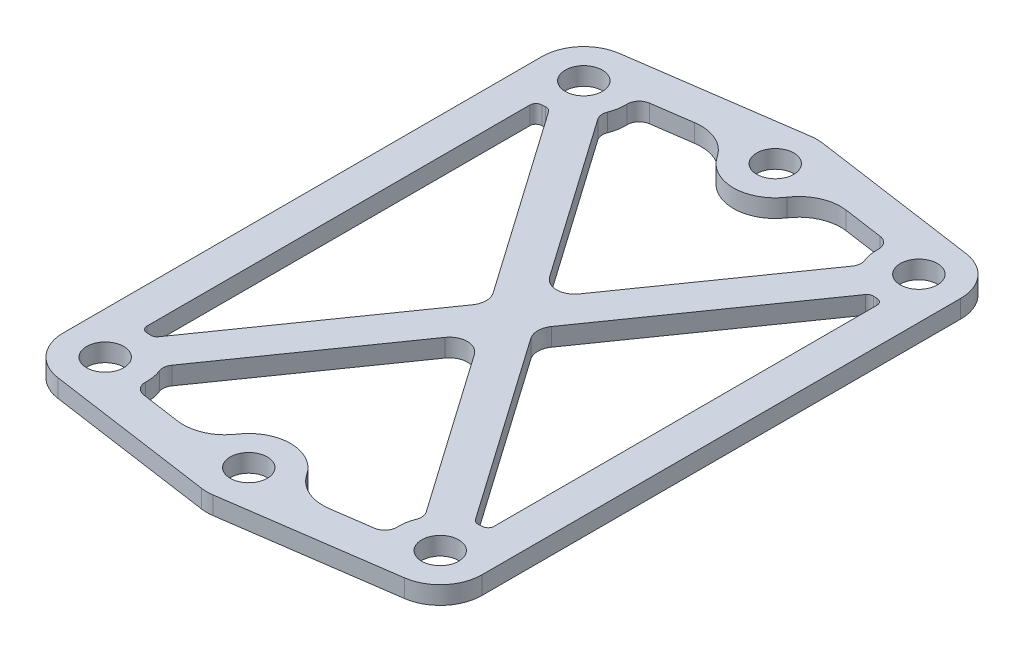
from build123d import *

# Parameters (mm, degrees)
SKETCH_1_R      = 1.55
EXTRUDE_1_DEPTH = 1.5
FILLET_1_R      = 0.5
FILLET_2_R      = 1
FILLET_3_R      = 1.5
FILLET_4_R      = 3.5


with BuildPart() as part:
    # 草图1 → 凸台-拉伸1 (new body)
    with BuildSketch(Plane(origin=(0, 0, 0), x_dir=(1, 0, 0), z_dir=(0, 1, 0))):
        with BuildLine():
            ThreePointArc((14.494974747, -23.464823228), (16.644088842, -22.293206095), (17.5, -20))
            Line((17.5, -20), (17.5, 20))
            ThreePointArc((17.5, 20), (16.644088842, 22.293206095), (14.494974747, 23.464823228))
            Line((14.494974747, 23.464823228), (0.494974747, 25.464823228))
            ThreePointArc((0.494974747, 25.464823228), (0, 25.5), (-0.494974747, 25.464823228))
            Line((-0.494974747, 25.464823228), (-14.494974747, 23.464823228))
            ThreePointArc((-14.494974747, 23.464823228), (-16.644088842, 22.293206095), (-17.5, 20))
            Line((-17.5, 20), (-17.5, -20))
            ThreePointArc((-17.5, -20), (-16.644088842, -22.293206095), (-14.494974747, -23.464823228))
            Line((-14.494974747, -23.464823228), (-0.494974747, -25.464823228))
            ThreePointArc((-0.494974747, -25.464823228), (0, -25.5), (0.494974747, -25.464823228))
            Line((0.494974747, -25.464823228), (14.494974747, -23.464823228))
        make_face()
        with BuildLine():
            Line((-10.957704959, -18.269554716), (0, -2.615690489))
            Line((0, -2.615690489), (10.957704959, -18.269554716))
            ThreePointArc((10.957704959, -18.269554716), (10.523504332, -19.595058191), (10.641425038, -20.984872695))
            Line((10.641425038, -20.984872695), (3.499996318, -22.005076798))
            ThreePointArc((3.499996318, -22.005076798), (0, -18.5), (-3.499996318, -22.005076798))
            Line((-3.499996318, -22.005076798), (-10.641425038, -20.984872695))
            ThreePointArc((-10.641425038, -20.984872695), (-10.523504332, -19.595058191), (-10.957704959, -18.269554716))
        make_face(mode=Mode.SUBTRACT)
        with BuildLine():
            ThreePointArc((14.5, -16.535898385), (13.957183203, -16.500261907), (13.41540072, -16.549167683))
            Line((13.41540072, -16.549167683), (1.830983342, 0))
            Line((1.830983342, 0), (13.41540072, 16.549167683))
            ThreePointArc((13.41540072, 16.549167683), (13.957183203, 16.500261907), (14.5, 16.535898385))
            Line((14.5, 16.535898385), (14.5, -16.535898385))
        make_face(mode=Mode.SUBTRACT)
        with BuildLine():
            Line((10.957704959, 18.269554716), (0, 2.615690489))
            Line((0, 2.615690489), (-10.957704959, 18.269554716))
            ThreePointArc((-10.957704959, 18.269554716), (-10.523504332, 19.595058191), (-10.641425038, 20.984872695))
            Line((-10.641425038, 20.984872695), (-3.499996318, 22.005076798))
            ThreePointArc((-3.499996318, 22.005076798), (0, 18.5), (3.499996318, 22.005076798))
            Line((3.499996318, 22.005076798), (10.641425038, 20.984872695))
            ThreePointArc((10.641425038, 20.984872695), (10.523504332, 19.595058191), (10.957704959, 18.269554716))
        make_face(mode=Mode.SUBTRACT)
        with Locations(Location((-14, -20, 0), (0, 0, 270))):
            Circle(SKETCH_1_R, mode=Mode.SUBTRACT)
        with BuildLine():
            Line((-1.830983342, 0), (-13.41540072, -16.549167683))
            ThreePointArc((-13.41540072, -16.549167683), (-13.957183203, -16.500261907), (-14.5, -16.535898385))
            Line((-14.5, -16.535898385), (-14.5, 16.535898385))
            ThreePointArc((-14.5, 16.535898385), (-13.957183203, 16.500261907), (-13.41540072, 16.549167683))
            Line((-13.41540072, 16.549167683), (-1.830983342, 0))
        make_face(mode=Mode.SUBTRACT)
        with Locations(Location((-14, 20, 0), (0, 0, 270))):
            Circle(SKETCH_1_R, mode=Mode.SUBTRACT)
        with Locations(Location((0, 22, 0), (0, 0, 270))):
            Circle(SKETCH_1_R, mode=Mode.SUBTRACT)
        with Locations(Location((0, -22, 0), (0, 0, 270))):
            Circle(SKETCH_1_R, mode=Mode.SUBTRACT)
        with Locations(Location((14, -20, 0), (0, 0, 270))):
            Circle(SKETCH_1_R, mode=Mode.SUBTRACT)
        with Locations(Location((14, 20, 0), (0, 0, 270))):
            Circle(SKETCH_1_R, mode=Mode.SUBTRACT)
    extrude(amount=EXTRUDE_1_DEPTH)

    # 圆角1
    fillet_1_edges = [part.edges().sort_by_distance(p)[0] for p in [
        (-14.5, 0.75, -16.535898385),
        (-14.5, 0.75, 16.535898385),
        (-13.41540072, 0.75, 16.549167683),
        (-13.41540072, 0.75, -16.549167683),
        (13.41540072, 0.75, 16.549167683),
        (14.5, 0.75, 16.535898385),
        (14.5, 0.75, -16.535898385),
        (13.41540072, 0.75, -16.549167683),
    ]]
    fillet(fillet_1_edges, radius=FILLET_1_R)

    # 圆角2
    fillet_2_edges = [part.edges().sort_by_distance(p)[0] for p in [
        (-10.957704959, 0.75, 18.269554716),
        (-10.641425038, 0.75, 20.984872695),
        (10.641425038, 0.75, 20.984872695),
        (10.957704959, 0.75, 18.269554716),
        (-10.641425038, 0.75, -20.984872695),
        (-10.957704959, 0.75, -18.269554716),
        (10.957704959, 0.75, -18.269554716),
        (10.641425038, 0.75, -20.984872695),
    ]]
    fillet(fillet_2_edges, radius=FILLET_2_R)

    # 圆角3
    fillet_3_edges = [part.edges().sort_by_distance(p)[0] for p in [
        (-1.830983342, 0.75, 0),
        (0, 0.75, 2.615690489),
        (1.830983342, 0.75, 0),
        (0, 0.75, -2.615690489),
    ]]
    fillet(fillet_3_edges, radius=FILLET_3_R)

    # 圆角4
    fillet_4_edges = [part.edges().sort_by_distance(p)[0] for p in [
        (-3.499996318, 0.75, 22.005076798),
        (3.499996318, 0.75, 22.005076798),
        (3.499996318, 0.75, -22.005076798),
        (-3.499996318, 0.75, -22.005076798),
    ]]
    fillet(fillet_4_edges, radius=FILLET_4_R)


solid = part.part
